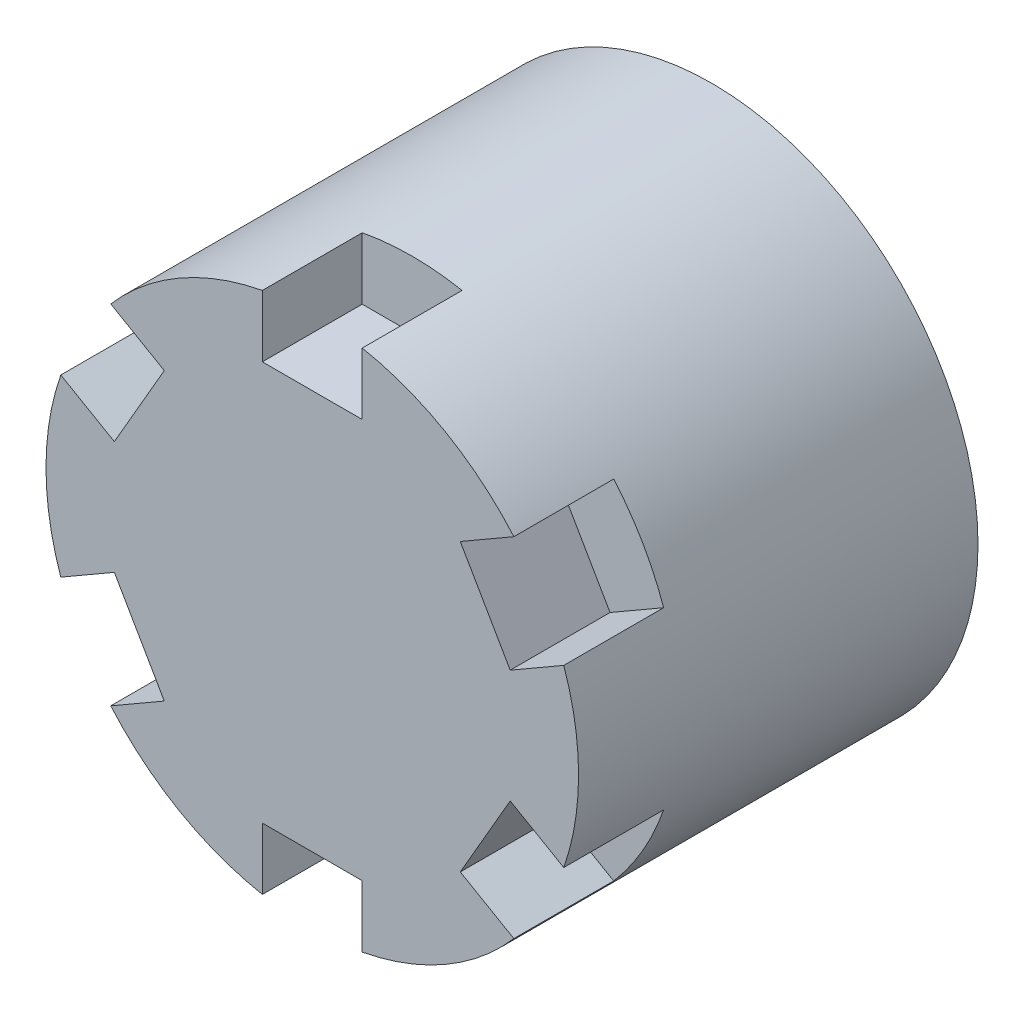
from build123d import *

# Parameters (mm, degrees)
SKETCH_2_R          = 40
EXTRUDE_1_DEPTH     = 60
SKETCH_1_R          = 19.5
CUT_EXTRUDE_1_DEPTH = 40
CUT_EXTRUDE_START   = -15
CUT_EXTRUDE_2_DEPTH = 15
SKETCH_4_W          = 20
SKETCH_4_H          = 7.082368082
CUT_EXTRUDE_3_DEPTH = 30


with BuildPart() as part:
    # 草图2 → 凸台-拉伸1 (new body)
    with BuildSketch(Plane.XY):
        Circle(SKETCH_2_R)
    extrude(amount=EXTRUDE_1_DEPTH)

    # 草图1 → 切除-拉伸1 (cut)
    with BuildSketch(Plane.XY):
        Circle(SKETCH_1_R)
    extrude(amount=CUT_EXTRUDE_1_DEPTH, mode=Mode.SUBTRACT)

    # 草图3 → 切除-拉伸2 (cut)
    with BuildSketch(Plane.XY.offset(60).offset(CUT_EXTRUDE_START)):
        with BuildLine():
            Line((22.230762114, 21.495190528), (29.730762114, 8.504809472))
            Line((29.730762114, 8.504809472), (37.776643972, 13.150101528))
            ThreePointArc((37.776643972, 13.150101528), (34.641016151, 20), (30.276643972, 26.140482585))
            Line((30.276643972, 26.140482585), (22.230762114, 21.495190528))
        make_face()
        with BuildLine():
            Line((-7.5, 39.290584114), (-7.5, 30))
            Line((-7.5, 30), (7.5, 30))
            Line((7.5, 30), (7.5, 39.290584114))
            ThreePointArc((7.5, 39.290584114), (0, 40), (-7.5, 39.290584114))
        make_face()
        with BuildLine():
            Line((29.730762114, -8.504809472), (22.230762114, -21.495190528))
            Line((22.230762114, -21.495190528), (30.276643972, -26.140482585))
            ThreePointArc((30.276643972, -26.140482585), (34.641016151, -20), (37.776643972, -13.150101528))
            Line((37.776643972, -13.150101528), (29.730762114, -8.504809472))
        make_face()
        with BuildLine():
            Line((7.5, -30), (-7.5, -30))
            Line((-7.5, -30), (-7.5, -39.290584114))
            ThreePointArc((-7.5, -39.290584114), (0, -40), (7.5, -39.290584114))
            Line((7.5, -39.290584114), (7.5, -30))
        make_face()
        with BuildLine():
            Line((-22.230762114, -21.495190528), (-29.730762114, -8.504809472))
            Line((-29.730762114, -8.504809472), (-37.776643972, -13.150101528))
            ThreePointArc((-37.776643972, -13.150101528), (-34.641016151, -20), (-30.276643972, -26.140482585))
            Line((-30.276643972, -26.140482585), (-22.230762114, -21.495190528))
        make_face()
        with BuildLine():
            Line((-29.730762114, 8.504809472), (-22.230762114, 21.495190528))
            Line((-22.230762114, 21.495190528), (-30.276643972, 26.140482585))
            ThreePointArc((-30.276643972, 26.140482585), (-34.641016151, 20), (-37.776643972, 13.150101528))
            Line((-37.776643972, 13.150101528), (-29.730762114, 8.504809472))
        make_face()
    extrude(amount=CUT_EXTRUDE_2_DEPTH, mode=Mode.SUBTRACT)

    # 草图4 → 切除-拉伸3 (cut)
    with BuildSketch(Plane(origin=(0, 0, 0), x_dir=(-1, 0, 0), z_dir=(0, 0, -1))):
        with Locations((0, 19.458815959)):
            Rectangle(SKETCH_4_W, SKETCH_4_H)
    extrude(amount=-CUT_EXTRUDE_3_DEPTH, mode=Mode.SUBTRACT)


solid = part.part
